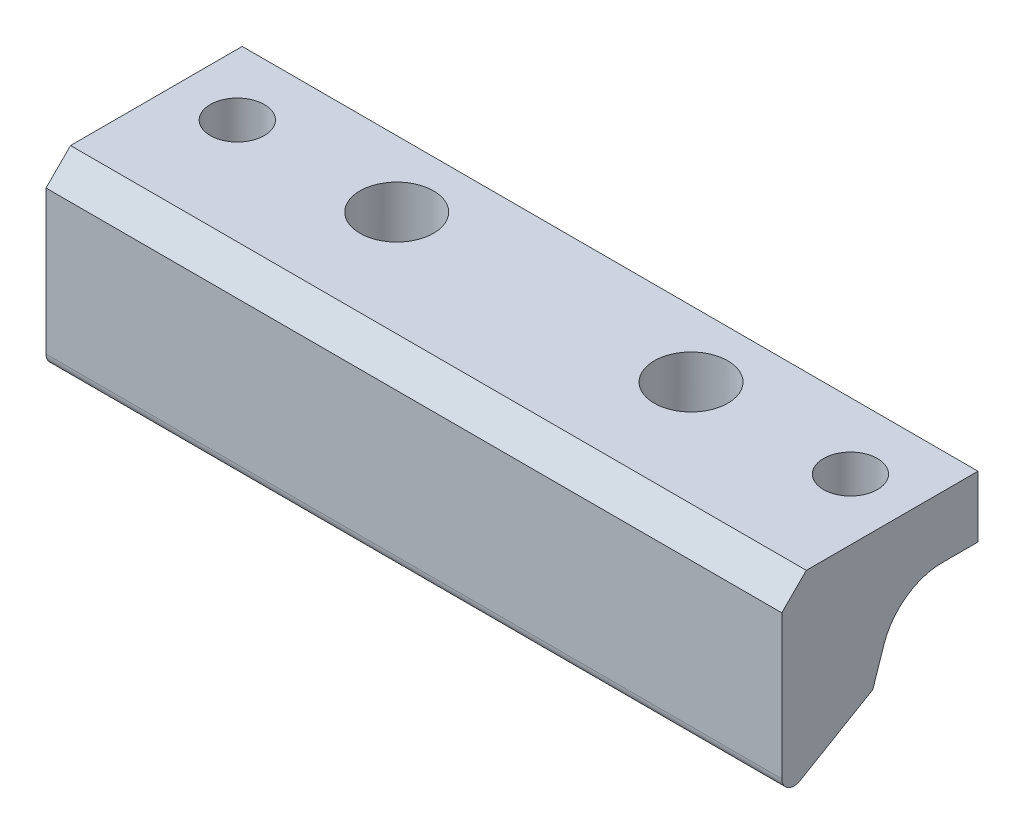
SolidWorks part; units mm, degrees
material "PEEK"
ref_plane "前视基准面" through (0, 0, 0) normal (0, 0, 1) x (1, 0, 0)
ref_plane "上视基准面" through (0, 0, 0) normal (0, 1, 0) x (1, 0, 0)
ref_plane "右视基准面" through (0, 0, 0) normal (1, 0, 0) x (0, 0, -1)
sketch "草图2" plane through (15, 0, 0) normal (1, 0, 0) x (0, 0, -1)
  line L0 (0, -3.5) -> (1, -2.5)
  line L1 (0, -3.5) -> (0, -9.3628)
  line L3 (0.7519, -9.7947) -> (3.7103, -8.069)
  line L4 (3.7103, -8.069) -> (4.1635, -6.7094)
  line L5 (8, -5) -> (6.5352, -5)
  line L6 (8, -5) -> (8, -2.5)
  line L7 (1, -2.5) -> (8, -2.5)
  arc A1 (6.5352, -5) -> (4.1635, -6.7094) centre (6.5352, -7.5) ccw
  arc A2 (0.7519, -9.7947) -> (0, -9.3628) centre (0.5, -9.3628) cw
extrude "凸台-拉伸1" add sketch "草图2" against normal up to surface (30 mm away)
hole_wizard "大小mm 暗销孔1" positions "草图9" profile "草图10" hole size "Ø3.0" standard "ISO" end condition through all
sketch "草图9" plane through (0, -2.5, 0) normal (0, 1, 0) x (1, 0, 0)
  point P0 (6, 5.3)
  point P3 (-6, 5.3)
sketch "草图10" plane through (6, -2.5, -5.3) normal (1, 0, 0) x (0, 0, 1)
  line L0 (0, 0) -> (0, 7.3628)
  line L1 (0, 7.3628) -> (1.5, 7.3628)
  line L2 (1.5, 7.3628) -> (1.5, 0)
  line L5 (1.5, 0) -> (0, 0)
  line L11 (0, -6.35) -> (0, 107.95) construction
  dimension "通孔孔直径" = 3
  dimension "通孔孔深度" = 7.3628
ref_plane "基准面1" through (0, -8.5, 0) normal (0, 1, 0) x (1, 0, 0)
sketch "草图13" plane through (0, -8.5, 0) normal (0, 1, 0) x (1, 0, 0)
  arc A1 (10.927, 6.5352) -> (14.073, 6.5352) centre (12.5, 5.3) ccw
  arc A2 (14.073, 6.5352) -> (10.927, 6.5352) centre (12.5, 4.9623) ccw
extrude "切除-拉伸1" cut sketch "草图13" along normal up to surface (3.5 mm away)
sketch "草图14" plane through (0, -5, 0) normal (0, -1, 0) x (1, 0, 0)
  arc A1 (-10.927, -6.5352) -> (-14.073, -6.5352) centre (-12.5, -5.3) ccw
  arc A2 (-14.073, -6.5352) -> (-10.927, -6.5352) centre (-12.5, -4.9623) ccw
extrude "切除-拉伸2" cut sketch "草图14" along normal up to surface (1.4211 mm away)
sketch "草图15" plane through (0, -5, 0) normal (0, -1, 0) x (1, 0, 0)
  circle A1 centre (12.5, -5.3) radius 1.1
  circle A3 centre (-12.5, -5.3) radius 1.1
extrude "切除-拉伸3" cut sketch "草图15" against normal blind 5
